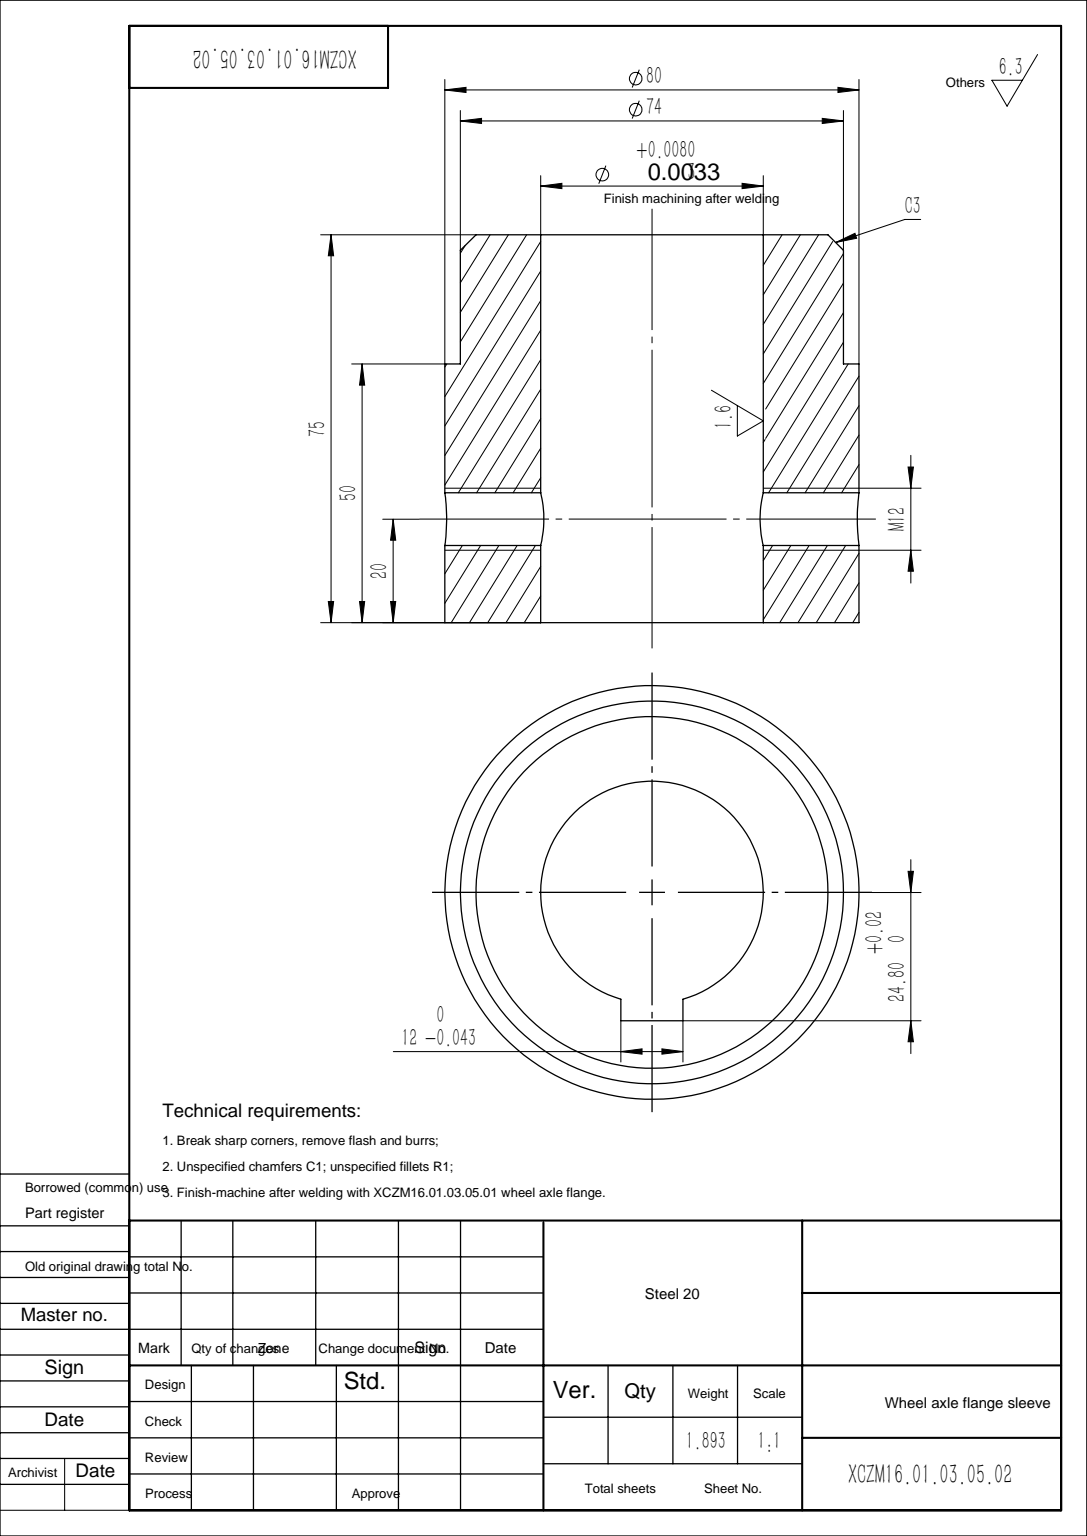
SolidWorks part; units mm, degrees
material "20 Steel"
ref_plane "Front Plane" through (0, 0, 0) normal (0, 0, 1) x (1, 0, 0)
ref_plane "Top Plane" through (0, 0, 0) normal (0, 1, 0) x (1, 0, 0)
ref_plane "Right Plane" through (0, 0, 0) normal (1, 0, 0) x (0, 0, -1)
sketch "Sketch2" plane through (0, 0, 0) normal (0, 0, 1) x (1, 0, 0)
  line L0 (0, 0) -> (40, 0)
  line L1 (40, 0) -> (40, 50)
  line L2 (40, 50) -> (37, 50)
  line L3 (37, 50) -> (37, 75)
  line L4 (37, 75) -> (0, 75)
  line L5 (0, 75) -> (0, -30.3154) construction
  line L6 (0, 0) -> (0, 75)
  line L7 (21.5, 75) -> (21.5, 0)
  dimension "D1" = 43
  dimension "D2" = 74
  dimension "D3" = 50
  dimension "D4" = 80
  dimension "D5" = 75
revolve "Revolve1" add sketch "Sketch2" angle 360 about L5
chamfer "Chamfer1" distance 3 angle 45 1 edges at (-37, 75, 0)
ref_plane "Plane1" through (40, 0, 0) normal (1, 0, 0) x (0, 0, -1)
hole_wizard "M12 Tapped Hole1" positions "Sketch4" profile "Sketch5" tap size "M12" standard "GB" end condition through all
sketch "Sketch4" plane through (40, 0, 0) normal (1, 0, 0) x (0, 0, -1)
  line L0 (0, 0) -> (0, 20) construction
  line L1 (-40, 0) -> (40, 0) construction
  point P0 (0, 20)
  dimension "D1" = 20
sketch "Sketch5" plane through (40, 20, 0) normal (0, 1, 0) x (0, 0, -1)
  line L0 (0, 0) -> (0, 80)
  line L1 (0, 80) -> (5.1, 80)
  line L2 (5.1, 80) -> (5.1, 0)
  line L5 (5.1, 0) -> (0, 0)
  line L11 (0, -6.35) -> (0, 107.95) construction
  dimension "通孔螺纹孔钻头直径" = 10.2
  dimension "通孔螺纹孔钻头深度" = 80
cosmetic thread "Hole Cosmetic Thread1" parameters "D2"=12
sketch "Sketch6" plane through (0, 75, 0) normal (0, 1, 0) x (1, 0, 0)
  line L0 (0, -21.5) -> (0, 0) construction
  line L1 (6, -24.8) -> (-6, -24.8)
  line L2 (6, -24.8) -> (6, -18.2)
  line L3 (6, -18.2) -> (-6, -18.2)
  line L4 (-6, -24.8) -> (-6, -18.2)
  line L5 (6, -24.8) -> (-6, -18.2) construction
  line L6 (6, -18.2) -> (-6, -24.8) construction
  circle A0 centre (0, 0) radius 21.5 construction
  point P0 (0, -21.5)
  dimension "D1" = 12
  dimension "D2" = 24.8
extrude "Cut-Extrude1" cut sketch "Sketch6" against normal up to next
